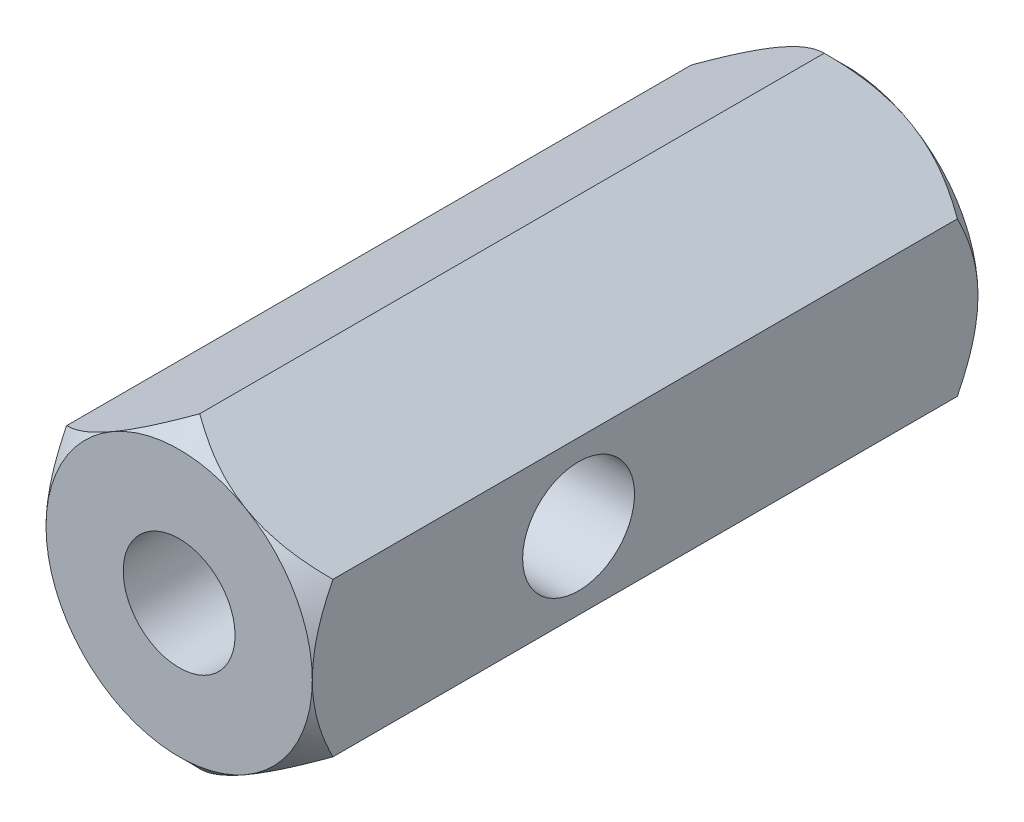
from build123d import *

# Parameters (mm, degrees)
BOSS_EXTRUDE1_DEPTH   = 25
M5_TAPPED_HOLE3_D     = 4.2
M5_TAPPED_HOLE3_DEPTH = 10
M5_TAPPED_HOLE3_TIP   = 1.2618073
M4_TAPPED_HOLE1_D     = 3.3
M4_TAPPED_HOLE1_DEPTH = 9
M4_TAPPED_HOLE1_TIP   = 0.991420021
SKETCH7_W             = 2.1
SKETCH7_H             = 5


with BuildPart() as part:
    # Sketch1 → Boss-Extrude1 (new body)
    with BuildSketch(Plane.XY):
        Polygon((0, 5.773502692), (-5, 2.886751346), (-5, -2.886751346), (0, -5.773502692), (5, -2.886751346), (5, 2.886751346), align=None)
    extrude(amount=BOSS_EXTRUDE1_DEPTH)

    # M5 Tapped Hole3
    with Locations(Plane.XY.offset(25)):
        with Locations((0, 0)):
            Hole(M5_TAPPED_HOLE3_D / 2, depth=M5_TAPPED_HOLE3_DEPTH)
            with Locations((0, 0, -(M5_TAPPED_HOLE3_DEPTH + M5_TAPPED_HOLE3_TIP / 2))):  # 118° drill point
                Cone(0, M5_TAPPED_HOLE3_D / 2, M5_TAPPED_HOLE3_TIP, mode=Mode.SUBTRACT)

    # M4 Tapped Hole1
    with Locations(Plane(origin=(0, 0, 0), x_dir=(-1, 0, 0), z_dir=(0, 0, -1))):
        with Locations((0, 0)):
            Hole(M4_TAPPED_HOLE1_D / 2, depth=M4_TAPPED_HOLE1_DEPTH)
            with Locations((0, 0, -(M4_TAPPED_HOLE1_DEPTH + M4_TAPPED_HOLE1_TIP / 2))):  # 118° drill point
                Cone(0, M4_TAPPED_HOLE1_D / 2, M4_TAPPED_HOLE1_TIP, mode=Mode.SUBTRACT)

    # Sketch7 → M5 Tapped Hole2 (revolve, cut)
    with BuildSketch(Plane(origin=(0, 0, 15), x_dir=(0, 0, 1), z_dir=(0, 1, 0))):
        with Locations((1.05, 2.5)):
            Rectangle(SKETCH7_W, SKETCH7_H)
    revolve(axis=Axis((-6.35, 0, 15), (1, 0, 0)), mode=Mode.SUBTRACT)

    # Sketch8 → Cut-Revolve1 (revolve, cut)
    with BuildSketch(Plane(origin=(0, 0, 0), x_dir=(0, 0, -1), z_dir=(1, 0, 0)), mode=Mode.PRIVATE) as cut_revolve1_sk:
        Polygon((-25, 5), (-25, 5.773502692), (-24.226497308, 5.773502692), align=None)
        Polygon((0, 5), (0, 5.773502692), (-0.773502692, 5.773502692), align=None)
    revolve(cut_revolve1_sk.sketch.rotate(Axis((0, 0, 25), (0, 0, -1)), 90), axis=Axis((0, 0, 25), (0, 0, -1)), mode=Mode.SUBTRACT)


solid = part.part
